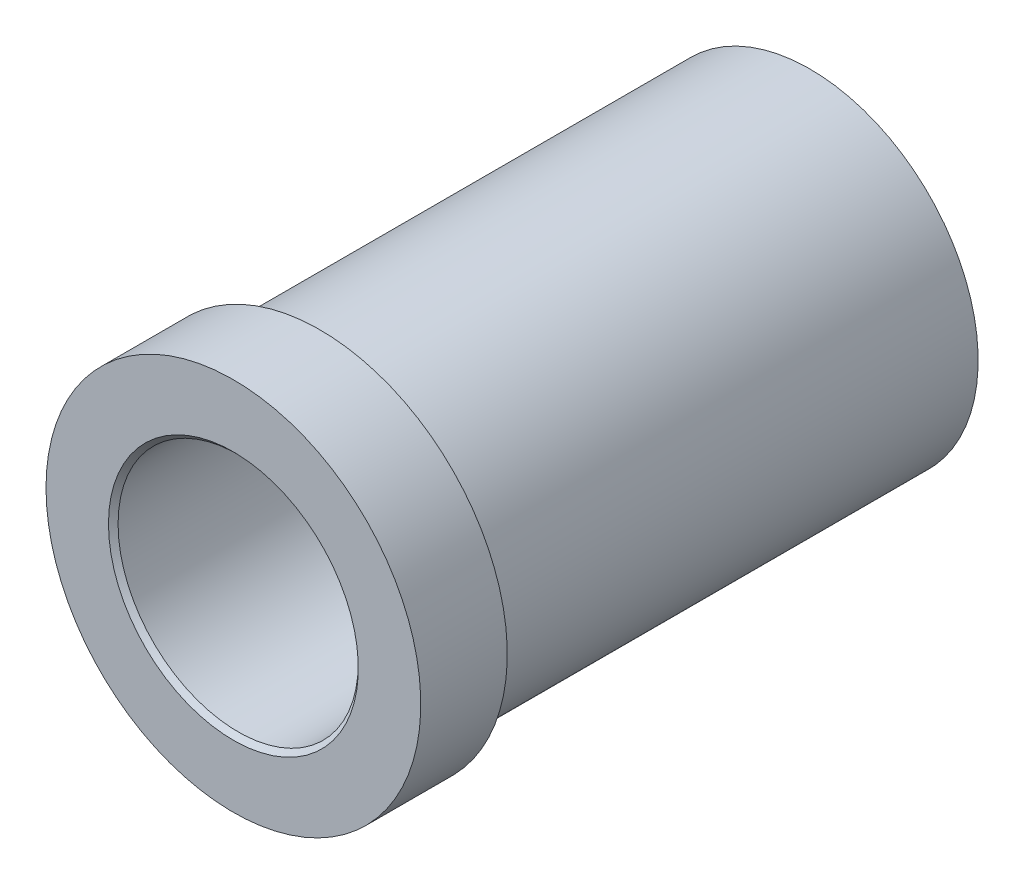
from build123d import *


with BuildPart() as part:
    # Sketch1 → Revolve1 (revolve)
    with BuildSketch(Plane.XZ, mode=Mode.PRIVATE) as revolve1_sk:
        Polygon((19.5, 0), (19.5, 9), (13, 9), (12.5, 8.5), (12.5, -50.5), (13, -51), (17.5, -51), (17.5, 0), align=None)
    revolve(revolve1_sk.sketch.rotate(Axis((0, 0, 9), (0, 0, -1)), 180), axis=Axis((0, 0, 9), (0, 0, -1)))


solid = part.part
